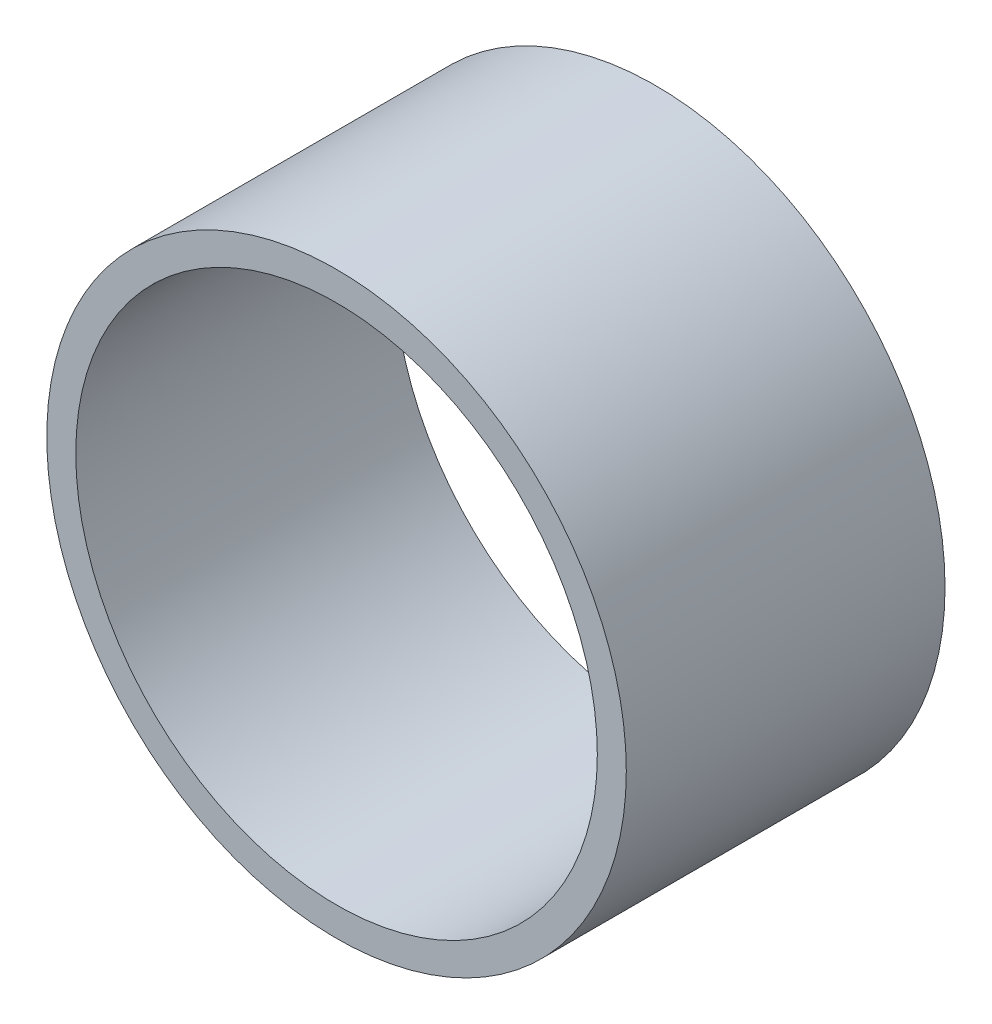
from build123d import *

# Parameters (mm, degrees)
SKETCH1_R           = 40
SKETCH1_R_2         = 36
BOSS_EXTRUDE1_DEPTH = 44


with BuildPart() as part:
    # Sketch1 → Boss-Extrude1 (new body)
    with BuildSketch(Plane.XY):
        with Locations((-1060, 0)):
            Circle(SKETCH1_R)
        with Locations((-1060, 0)):
            Circle(SKETCH1_R_2, mode=Mode.SUBTRACT)
    extrude(amount=BOSS_EXTRUDE1_DEPTH)


solid = part.part
